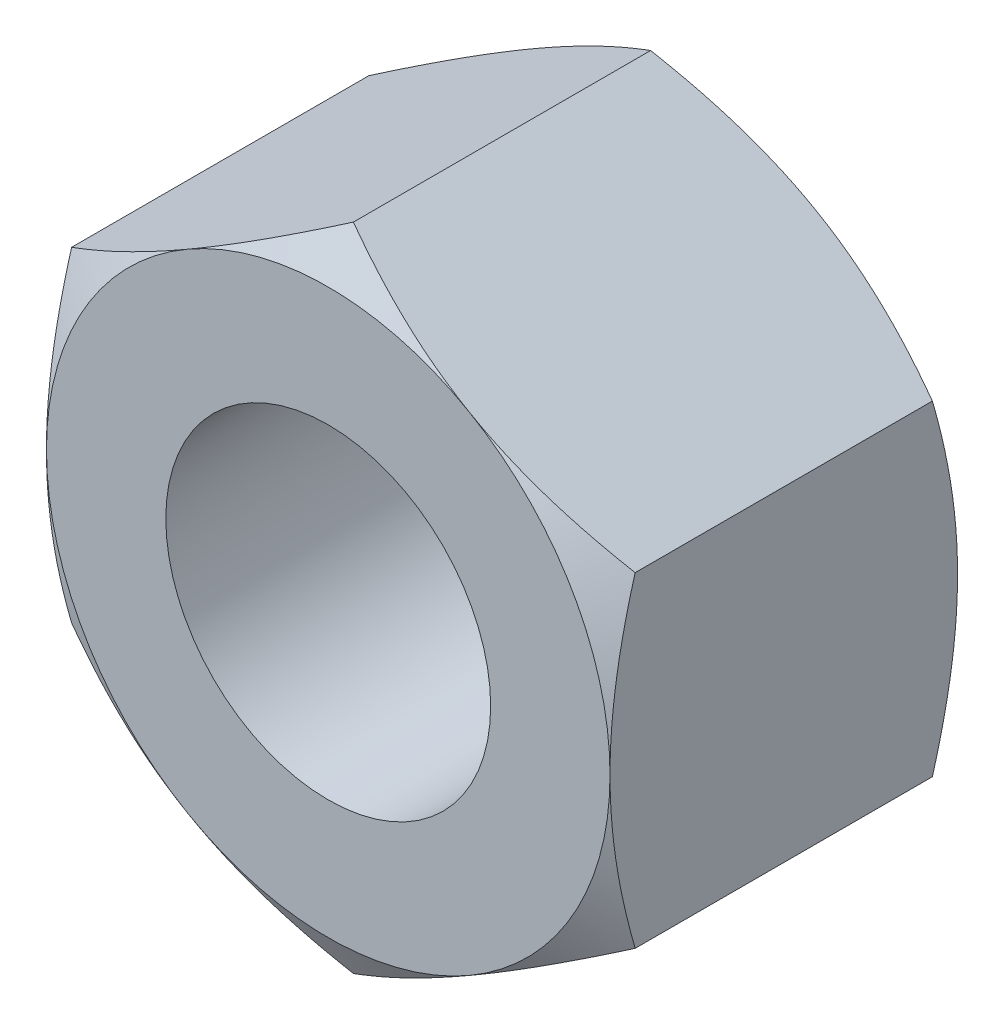
from build123d import *

# Parameters (mm, degrees)
SKETCH_1_R          = 6.9175
EXTRUDE_597_DEPTH   = 14.8
SKETCH_2_OUTSIDE_W  = 118.982
SKETCH_2_OUTSIDE_H  = 122.694
SKETCH_2_OUTSIDE_R  = 12
CUT_EXTRUDE_1_DEPTH = 24.559286916
CUT_EXTRUDE_1_DRAFT = -60
SKETCH_3_OUTSIDE_W  = 118.982
SKETCH_3_OUTSIDE_H  = 122.694
SKETCH_3_OUTSIDE_R  = 12
CUT_EXTRUDE_2_DEPTH = 24.559286916
CUT_EXTRUDE_2_DRAFT = -60


with BuildPart() as part:
    # 草图1 → Extrude 597 (new body)
    with BuildSketch(Plane.XY):
        Polygon((0, 13.856406461), (-12, 6.92820323), (-12, -6.92820323), (0, -13.856406461), (12, -6.92820323), (12, 6.92820323), align=None)
        Circle(SKETCH_1_R, mode=Mode.SUBTRACT)
    extrude(amount=EXTRUDE_597_DEPTH)


with BuildPart() as cut_extrude_1_tool:
    # 草图2 outside → 切除-拉伸1 (with draft: the straight prism first)
    with BuildSketch(Plane(origin=(0, 0, 0), x_dir=(-1, 0, 0), z_dir=(0, 0, -1))):
        Rectangle(SKETCH_2_OUTSIDE_W, SKETCH_2_OUTSIDE_H)
        Circle(SKETCH_2_OUTSIDE_R, mode=Mode.SUBTRACT)
    extrude(amount=-CUT_EXTRUDE_1_DEPTH)
    # 切除-拉伸1: the draft: its side faces are tilted about the plane it starts from
    cut_extrude_1_sides = [cut_extrude_1_tool.faces().sort_by_distance(p)[0] for p in [
        (0, -61.347, 12.279643458),
        (-59.491, 0, 12.279643458),
        (0, 61.347, 12.279643458),
        (59.491, 0, 12.279643458),
        (12, 0, 12.279643458),
    ]]
    draft(cut_extrude_1_sides, Plane(origin=(0, 0, 0), x_dir=(-1, 0, 0), z_dir=(0, 0, -1)), CUT_EXTRUDE_1_DRAFT)


with BuildPart() as part_1:
    add(part.part)

    # 切除-拉伸1: cut by cut_extrude_1_tool
    add(cut_extrude_1_tool.part, mode=Mode.SUBTRACT)


with BuildPart() as cut_extrude_2_tool:
    # 草图3 outside → 切除-拉伸2 (with draft: the straight prism first)
    with BuildSketch(Plane.XY.offset(14.8)):
        Rectangle(SKETCH_3_OUTSIDE_W, SKETCH_3_OUTSIDE_H)
        Circle(SKETCH_3_OUTSIDE_R, mode=Mode.SUBTRACT)
    extrude(amount=-CUT_EXTRUDE_2_DEPTH)
    # 切除-拉伸2: the draft: its side faces are tilted about the plane it starts from
    cut_extrude_2_sides = [cut_extrude_2_tool.faces().sort_by_distance(p)[0] for p in [
        (0, -61.347, 2.520356542),
        (59.491, 0, 2.520356542),
        (0, 61.347, 2.520356542),
        (-59.491, 0, 2.520356542),
        (-12, 0, 2.520356542),
    ]]
    draft(cut_extrude_2_sides, Plane.XY.offset(14.8), CUT_EXTRUDE_2_DRAFT)


with BuildPart() as part_2:
    add(part_1.part)

    # 切除-拉伸2: cut by cut_extrude_2_tool
    add(cut_extrude_2_tool.part, mode=Mode.SUBTRACT)


solid = part_2.part
